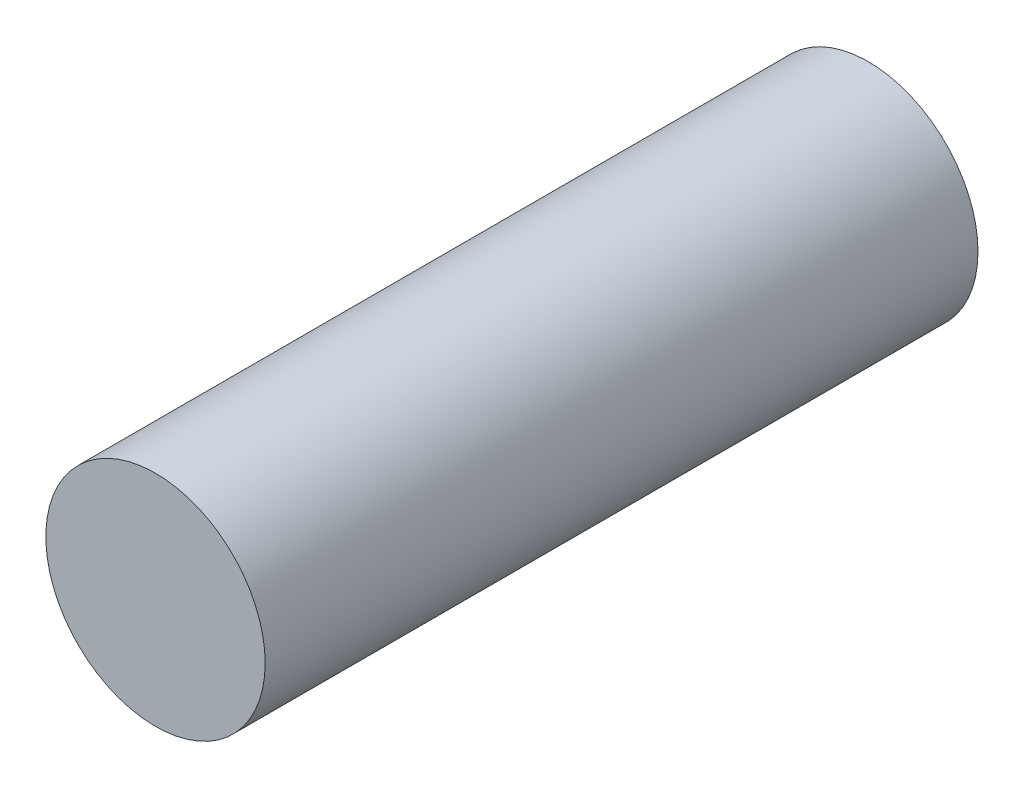
SolidWorks part; units mm, degrees
material "镀铬棒（硬）"
ref_plane "前视基准面" through (0, 0, 0) normal (0, 0, 1) x (1, 0, 0)
ref_plane "上视基准面" through (0, 0, 0) normal (0, 1, 0) x (1, 0, 0)
ref_plane "右视基准面" through (0, 0, 0) normal (1, 0, 0) x (0, 0, -1)
sketch "草图1" plane through (0, 0, 0) normal (0, 0, 1) x (1, 0, 0)
  circle A0 centre (0, 0) radius 10
  dimension "D1" = 20
extrude "凸台-拉伸1" add sketch "草图1" along normal blind 65
